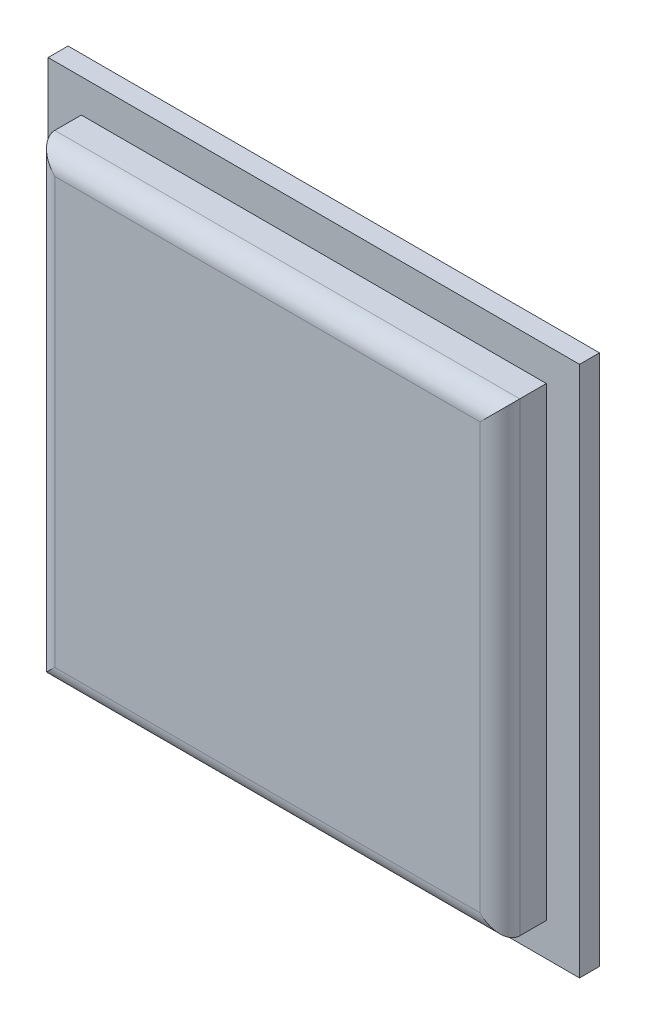
from build123d import *

# Parameters (mm, degrees)
SKETCH1_W           = 80
SKETCH1_H           = 80
BOSS_EXTRUDE1_DEPTH = 3
SKETCH2_W           = 70
SKETCH2_H           = 70
BOSS_EXTRUDE2_DEPTH = 7
FILLET1_R           = 3


with BuildPart() as part:
    # Sketch1 → Boss-Extrude1 (new body)
    with BuildSketch(Plane.XY):
        Rectangle(SKETCH1_W, SKETCH1_H)
    extrude(amount=BOSS_EXTRUDE1_DEPTH)

    # Sketch2 → Boss-Extrude2 (add)
    with BuildSketch(Plane.XY.offset(3)):
        Rectangle(SKETCH2_W, SKETCH2_H)
    extrude(amount=BOSS_EXTRUDE2_DEPTH)

    # Fillet1
    fillet1_edges = [part.edges().sort_by_distance(p)[0] for p in [
        (35, 0, 10),
        (0, 35, 10),
        (-35, 0, 10),
        (0, -35, 10),
    ]]
    fillet(fillet1_edges, radius=FILLET1_R)


solid = part.part
